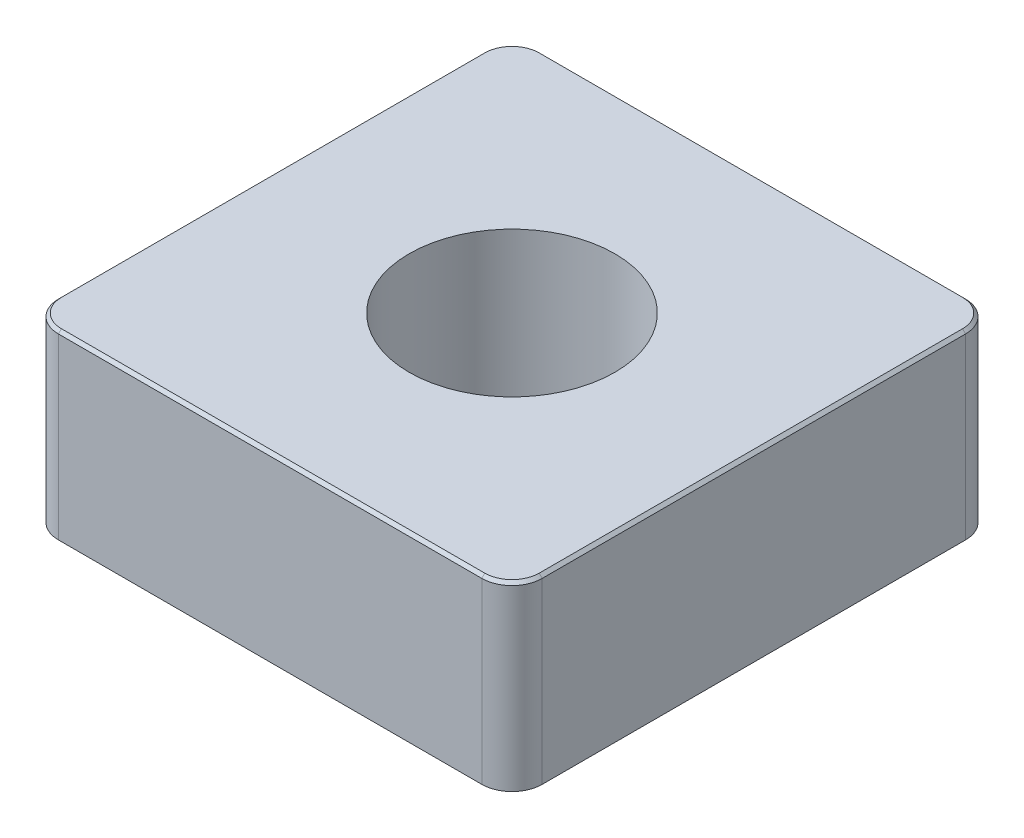
SolidWorks part; units mm, degrees
ref_plane "Front Plane" through (0, 0, 0) normal (0, 0, 1) x (1, 0, 0)
ref_plane "Top Plane" through (0, 0, 0) normal (0, 1, 0) x (1, 0, 0)
ref_plane "Right Plane" through (0, 0, 0) normal (1, 0, 0) x (0, 0, -1)
ref_plane "Plane4" through (0, 30, 0) normal (0, 1, 0) x (1, 0, 0)
sketch "Sketch1" plane through (0, 30, 0) normal (0, 1, 0) x (1, 0, 0)
  line L0 (-40, -40) -> (40, -40)
  line L1 (40, -40) -> (40, 40)
  line L2 (40, 40) -> (-40, 40)
  line L3 (-40, 40) -> (-40, -40)
  dimension "D1" = 80
extrude "Boss-Extrude1" add sketch "Sketch1" against normal blind 30
hole_wizard "M36x2.0 Tapped Hole1" positions "Sketch3" profile "Sketch2" tap size "M36x2.0" standard "ANSI Metric" end condition through all
sketch "Sketch3" plane through (0, 30, 0) normal (0, 1, 0) x (1, 0, 0)
  point P0 (0, 0)
sketch "Sketch2" plane through (0, 30, 0) normal (1, 0, 0) x (0, 0, 1)
  line L0 (0, 0) -> (0, 30)
  line L1 (0, 30) -> (17, 30)
  line L2 (17, 30) -> (17, 0)
  line L5 (17, 0) -> (0, 0)
  line L11 (0, -6.35) -> (0, 107.95) construction
  dimension "螺纹线主直径" = 34
  dimension "通孔螺纹孔钻头深度" = 30
fillet "Fillet1" radius 5 4 edges at (40, 15, 40) (-40, 15, 40) (40, 15, -40) (-40, 15, -40)
chamfer "Chamfer1" distance 0.5 angle 45 8 edges at (0, 30, -40) (38.5355, 30, -38.5355) (-38.5355, 30, -38.5355) (40, 30, 0) (-40, 30, 0) (38.5355, 30, 38.5355) (-38.5355, 30, 38.5355) (0, 30, 40)
